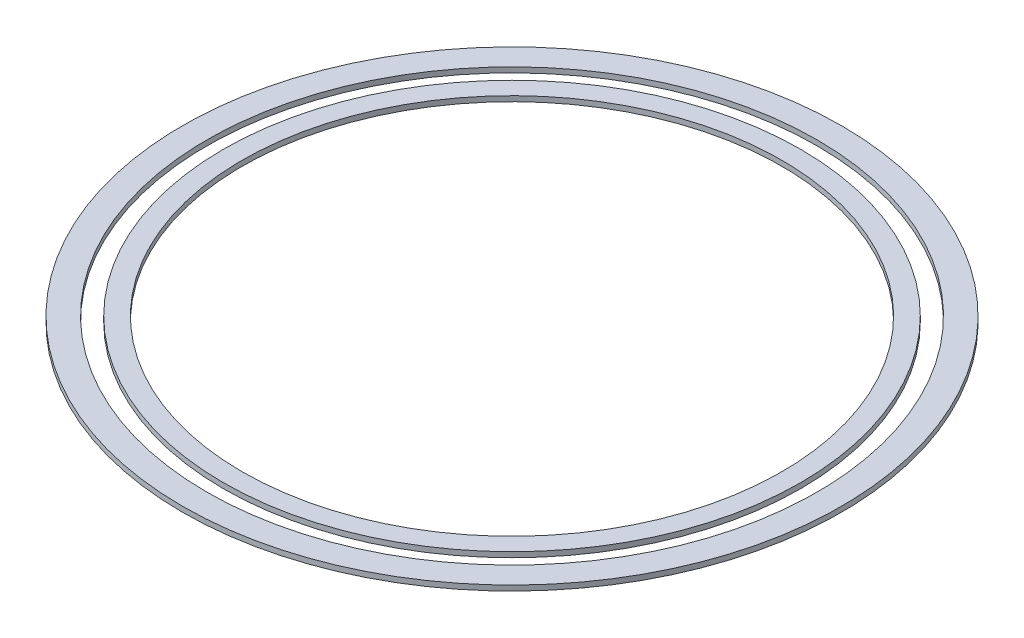
from build123d import *

# Parameters (mm, degrees)
SKETCH1_W   = 5.524909439
SKETCH1_H   = 1.185499442
SKETCH1_W_2 = 4.266122689


with BuildPart() as part:
    # Sketch1 → Revolve1 (revolve)
    with BuildSketch(Plane.XY, mode=Mode.PRIVATE) as revolve1_sk:
        with Locations((71.733252241, 136.907250279)):
            Rectangle(SKETCH1_W, SKETCH1_H)
        with Locations((63.128768306, 136.907250279)):
            Rectangle(SKETCH1_W_2, SKETCH1_H)
    revolve(revolve1_sk.sketch.rotate(Axis((0, 0, 0), (0, -1, 0)), 90), axis=Axis((0, 0, 0), (0, -1, 0)))


solid = part.part
